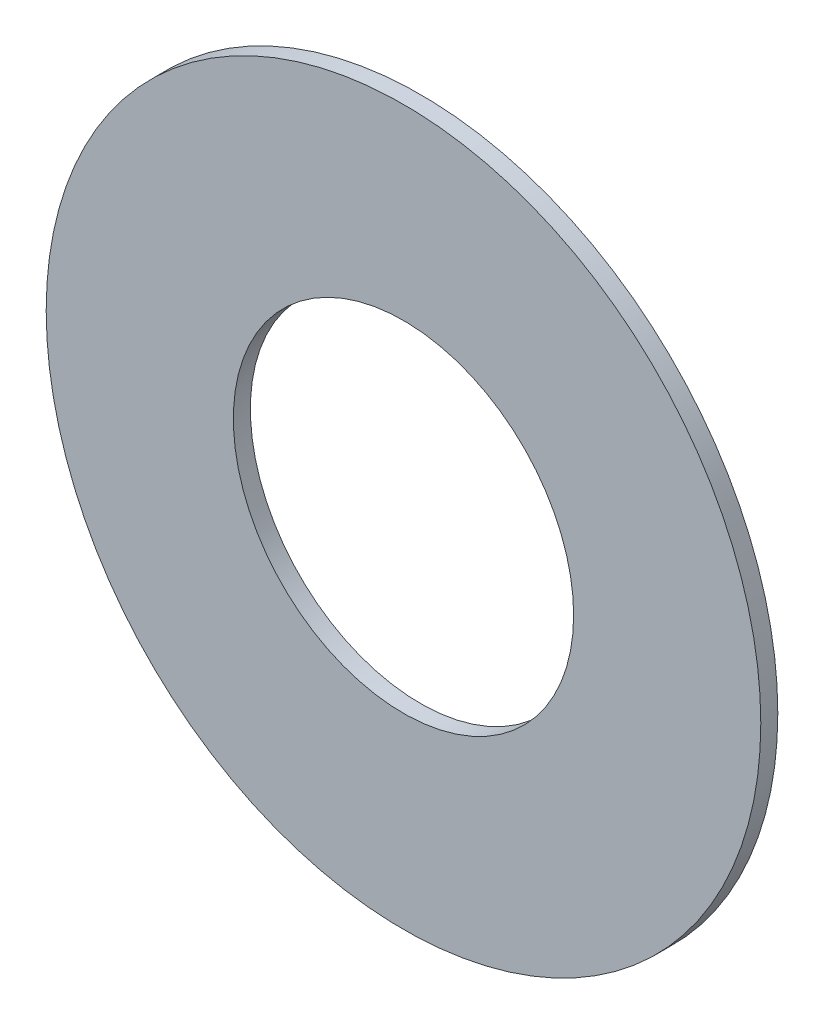
SolidWorks part; units mm, degrees
material "1.4000 (X6Cr13)"
ref_plane "Front Plane" through (0, 0, 0) normal (0, 0, 1) x (1, 0, 0)
ref_plane "Top Plane" through (0, 0, 0) normal (0, 1, 0) x (1, 0, 0)
ref_plane "Right Plane" through (0, 0, 0) normal (1, 0, 0) x (0, 0, -1)
sketch "Sketch1" plane through (0, 0, 0) normal (0, 0, 1) x (1, 0, 0)
  circle A0 centre (-121.5312, 115.619) radius 10.5
  circle A2 centre (-121.5312, 115.619) radius 5
  dimension "D1" = 21
extrude "Boss-Extrude1" add sketch "Sketch1" along normal blind 0.5
